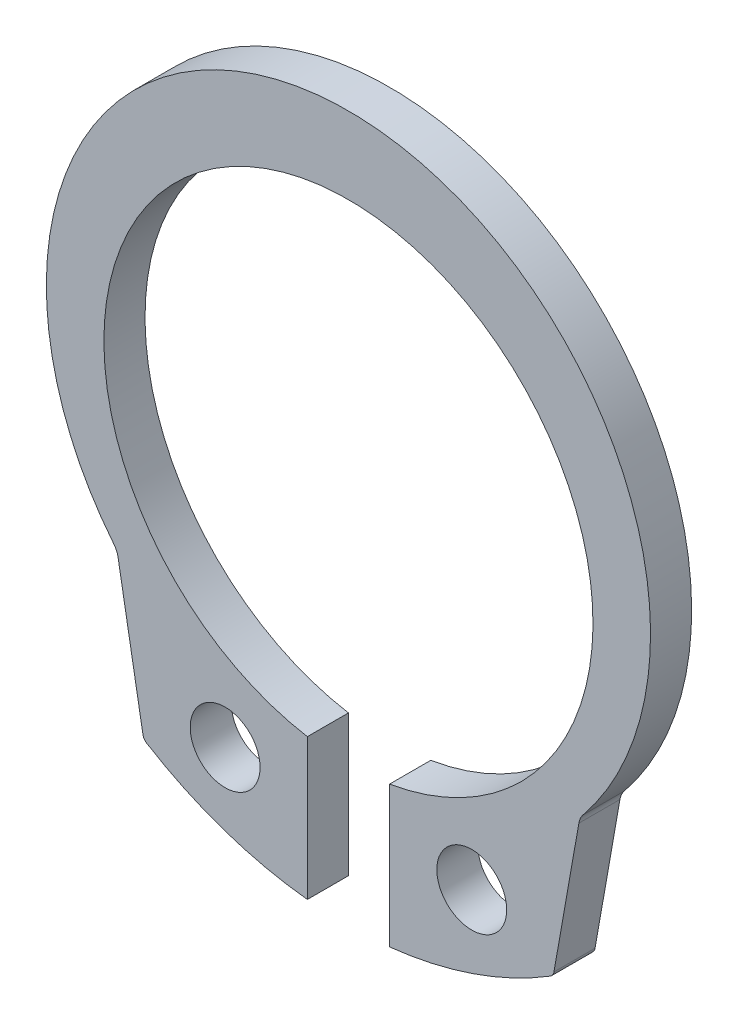
from build123d import *

# Parameters (mm, degrees)
BASE_EXTRUDE_DEPTH      = 0.5
BASE_EXTRUDE_DEPTH_BACK = 0.5
SKETCH1_R               = 0.85


with BuildPart() as part:
    # Sketch1 → Base-Extrude (new, two sides: drawn at the far end of the back side and taken through both)
    with BuildSketch(Plane.XY.offset(-BASE_EXTRUDE_DEPTH_BACK)):
        with BuildLine():
            Line((-1, -6.335364439), (-1, -9.766370259))
            ThreePointArc((-1, -9.766370259), (-3.028831825, -9.315828269), (-4.908022896, -8.428254284))
            ThreePointArc((-4.908022896, -8.428254284), (-4.968516352, -8.37034995), (-5, -8.292753881))
            Line((-5, -8.292753881), (-5.605979842, -4.856071421))
            ThreePointArc((-5.605979842, -4.856071421), (-5.643449504, -4.735447058), (-5.709951634, -4.628061401))
            ThreePointArc((-5.709951634, -4.628061401), (0, 7.35), (5.709951634, -4.628061401))
            ThreePointArc((5.709951634, -4.628061401), (5.643449504, -4.735447058), (5.605979842, -4.856071421))
            Line((5.605979842, -4.856071421), (5, -8.292753881))
            ThreePointArc((5, -8.292753881), (4.968516352, -8.37034995), (4.908022896, -8.428254284))
            ThreePointArc((4.908022896, -8.428254284), (3.028831825, -9.315828269), (1, -9.766370259))
            Line((1, -9.766370259), (1, -6.335364439))
            ThreePointArc((1, -6.335364439), (0, 5.48), (-1, -6.335364439))
        make_face()
        with Locations((-3, -7.561544261)):
            Circle(SKETCH1_R, mode=Mode.SUBTRACT)
        with Locations(Location((3, -7.561544261, 0), (0, 0, 180))):
            Circle(SKETCH1_R, mode=Mode.SUBTRACT)
    extrude(amount=BASE_EXTRUDE_DEPTH + BASE_EXTRUDE_DEPTH_BACK)


solid = part.part
